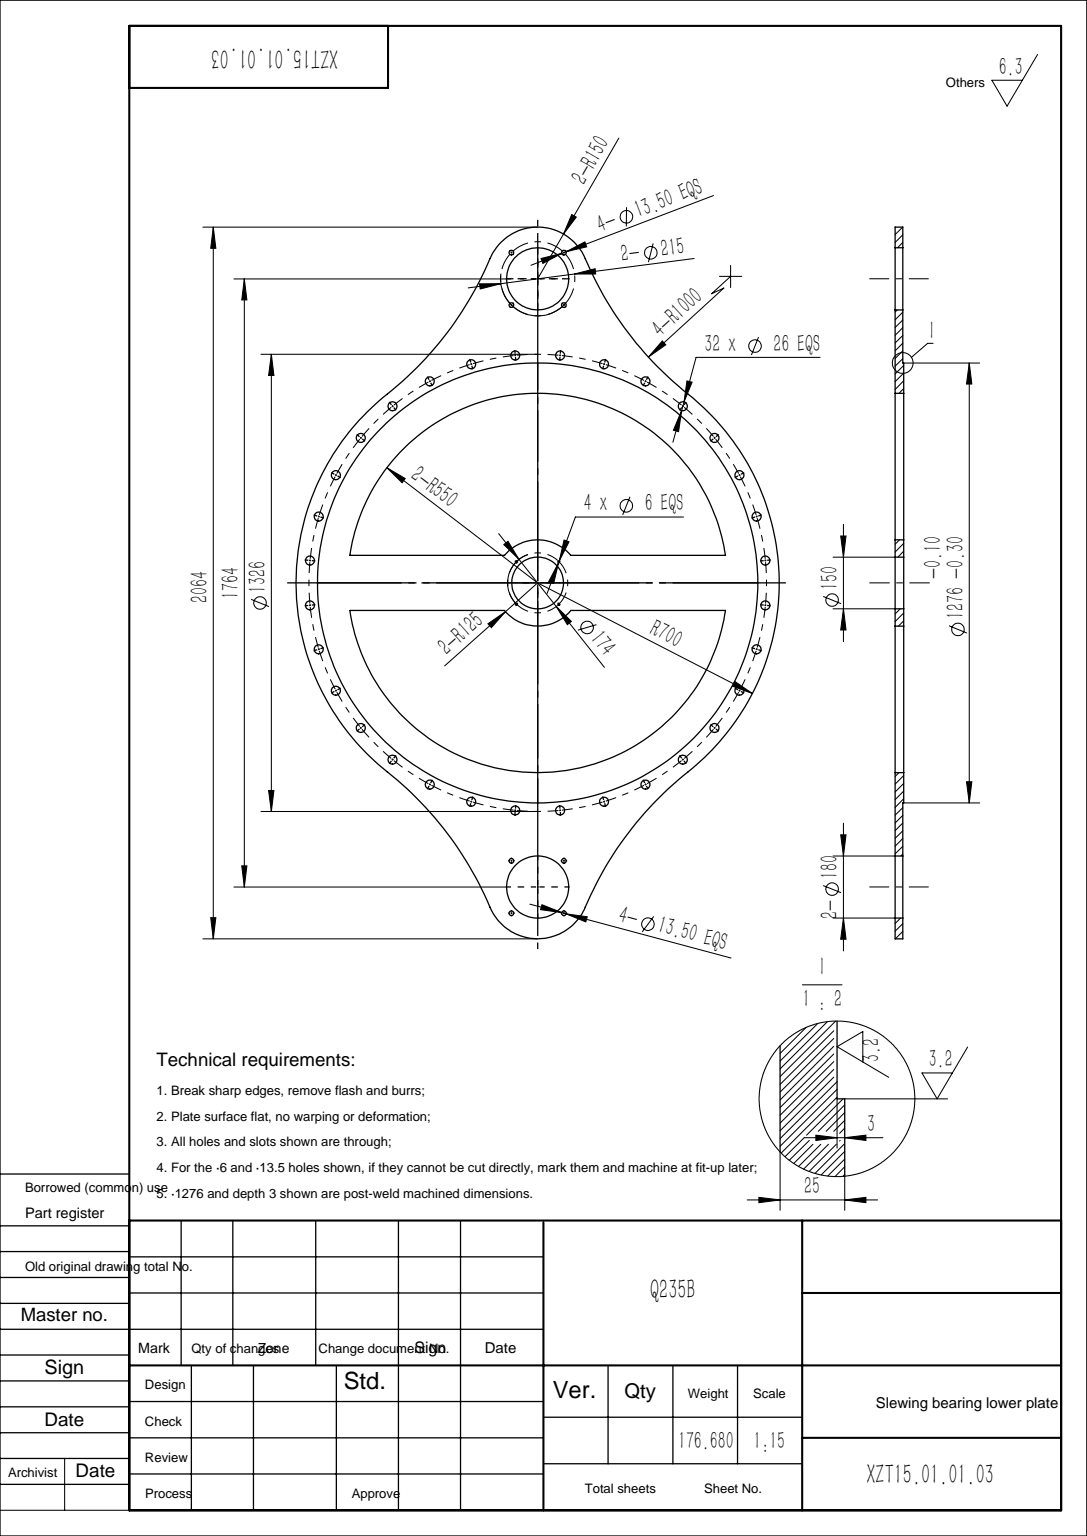
from build123d import *

# Parameters (mm, degrees)
SKETCH1_R                    = 75
SKETCH1_R_2                  = 90
BOSS_EXTRUDE1_DEPTH          = 25
SKETCH2_OUTSIDE_W            = 1900.828
SKETCH2_OUTSIDE_H            = 2564.828
SKETCH2_OUTSIDE_R            = 638
CUT_EXTRUDE1_DEPTH           = 3
F_24_5_24_5_DIAMETER_HOLE1_D = 26
F_6_0_6_DIAMETER_HOLE1_D     = 6
F_13_5_13_5_DIAMETER_HOLE1_D = 13.5


with BuildPart() as part:
    # Sketch1 → Boss-Extrude1 (new body)
    with BuildSketch(Plane(origin=(0, 0, 0), x_dir=(1, 0, 0), z_dir=(0, 1, 0))):
        with BuildLine():
            ThreePointArc((436.188742989, 547.484593838), (262.581338083, 725.275527763), (138.171589394, 940.383318545))
            ThreePointArc((138.171589394, 940.383318545), (0, 1032), (-138.171589394, 940.383318545))
            ThreePointArc((-138.171589394, 940.383318545), (-262.581338083, 725.275527763), (-436.188742989, 547.484593838))
            ThreePointArc((-436.188742989, 547.484593838), (-700, 0), (-436.188742989, -547.484593838))
            ThreePointArc((-436.188742989, -547.484593838), (-262.581338083, -725.275527763), (-138.171589394, -940.383318545))
            ThreePointArc((-138.171589394, -940.383318545), (0, -1032), (138.171589394, -940.383318545))
            ThreePointArc((138.171589394, -940.383318545), (262.581338083, -725.275527763), (436.188742989, -547.484593838))
            ThreePointArc((436.188742989, -547.484593838), (700, 0), (436.188742989, 547.484593838))
        make_face()
        with BuildLine():
            Line((544.150714417, 80), (96.046863561, 80))
            ThreePointArc((96.046863561, 80), (0, 125), (-96.046863561, 80))
            Line((-96.046863561, 80), (-544.150714417, 80))
            ThreePointArc((-544.150714417, 80), (0, 550), (544.150714417, 80))
        make_face(mode=Mode.SUBTRACT)
        with BuildLine():
            Line((-544.150714417, -80), (-96.046863561, -80))
            ThreePointArc((-96.046863561, -80), (0, -125), (96.046863561, -80))
            Line((96.046863561, -80), (544.150714417, -80))
            ThreePointArc((544.150714417, -80), (0, -550), (-544.150714417, -80))
        make_face(mode=Mode.SUBTRACT)
        with Locations(Location((0, 0, 0), (0, 0, 270))):
            Circle(SKETCH1_R, mode=Mode.SUBTRACT)
        with Locations(Location((0, 882, 0), (0, 0, 270))):
            Circle(SKETCH1_R_2, mode=Mode.SUBTRACT)
        with Locations(Location((0, -882, 0), (0, 0, 270))):
            Circle(SKETCH1_R_2, mode=Mode.SUBTRACT)
    extrude(amount=BOSS_EXTRUDE1_DEPTH)

    # Sketch2 outside → Cut-Extrude1 (cut)
    with BuildSketch(Plane(origin=(0, 25, 0), x_dir=(1, 0, 0), z_dir=(0, 1, 0))):
        Rectangle(SKETCH2_OUTSIDE_W, SKETCH2_OUTSIDE_H)
        with Locations(Location((0, 0, 0), (0, 0, 270))):
            Circle(SKETCH2_OUTSIDE_R, mode=Mode.SUBTRACT)
    extrude(amount=-CUT_EXTRUDE1_DEPTH, mode=Mode.SUBTRACT)

    # Ø24.5 (24.5) Diameter Hole1 (through all)
    with Locations(Plane(origin=(0, 22, 0), x_dir=(1, 0, 0), z_dir=(0, 1, 0))):
        with Locations((659.807473784, 64.985364038), (659.807473784, -64.985364038), (634.45144259, -192.45874102), (584.713798263, -312.536036516), (512.505930579, -420.6027474), (420.6027474, -512.505930579), (312.536036516, -584.713798263), (192.45874102, -634.45144259), (64.985364038, -659.807473784), (-64.985364038, -659.807473784), (-192.45874102, -634.45144259), (-312.536036516, -584.713798263), (-420.6027474, -512.505930579), (-512.505930579, -420.6027474), (-584.713798263, -312.536036516), (-634.45144259, -192.45874102), (-659.807473784, -64.985364038), (-659.807473784, 64.985364038), (-634.45144259, 192.45874102), (-584.713798263, 312.536036516), (-512.505930579, 420.6027474), (-420.6027474, 512.505930579), (-312.536036516, 584.713798263), (-192.45874102, 634.45144259), (-64.985364038, 659.807473784), (64.985364038, 659.807473784), (192.45874102, 634.45144259), (312.536036516, 584.713798263), (420.6027474, 512.505930579), (512.505930579, 420.6027474), (584.713798263, 312.536036516), (634.45144259, 192.45874102)):
            Hole(F_24_5_24_5_DIAMETER_HOLE1_D / 2)

    # Ø6.0 (6) Diameter Hole1 (through all)
    with Locations(Plane(origin=(0, 25, 0), x_dir=(1, 0, 0), z_dir=(0, 1, 0))):
        with Locations((-61.518289963, 61.518289963), (61.518289963, 61.518289963), (61.518289963, -61.518289963), (-61.518289963, -61.518289963)):
            Hole(F_6_0_6_DIAMETER_HOLE1_D / 2)

    # Ø13.5 (13.5) Diameter Hole1 (through all)
    with Locations(Plane(origin=(0, 22, 0), x_dir=(1, 0, 0), z_dir=(0, 1, 0))):
        with Locations((-76.013978978, 958.013978978), (76.013978978, 958.013978978), (76.013978978, 805.986021022), (-76.013978978, 805.986021022)):
            f_13_5_13_5_diameter_hole1 = Hole(F_13_5_13_5_DIAMETER_HOLE1_D / 2)

    # Mirror1: Ø13.5 (13.5) Diameter Hole1 across plane
    add(f_13_5_13_5_diameter_hole1.mirror(Plane.XY), mode=Mode.SUBTRACT)


solid = part.part
